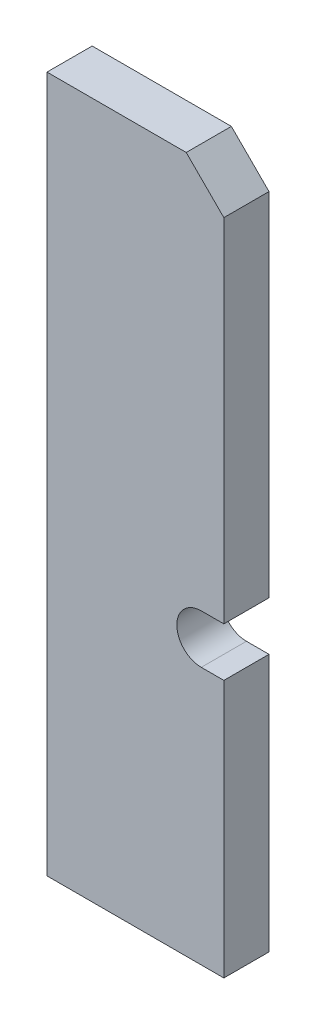
from build123d import *

# Parameters (mm, degrees)
SKETCH_1_W          = 47
SKETCH_1_H          = 185
EXTRUDE_1_DEPTH     = 6
CHAMFER_1_SIZE      = 10
CUT_EXTRUDE_2_REACH = 193.254


with BuildPart() as part:
    # 草图1 → 凸台-拉伸1 (new, symmetric)
    with BuildSketch(Plane.XY):
        with Locations((23.5, 92.5)):
            Rectangle(SKETCH_1_W, SKETCH_1_H)
    extrude(amount=EXTRUDE_1_DEPTH, both=True)

    # 倒角1
    chamfer_1_edges = [part.edges().sort_by_distance(p)[0] for p in [
        (47, 185, 0),
    ]]
    chamfer(chamfer_1_edges, length=CHAMFER_1_SIZE)

    # 草图3 → 切除-拉伸2 (cut, up to next)
    with BuildSketch(Plane(origin=(0, 0, -6), x_dir=(-1, 0, 0), z_dir=(0, 0, -1)), mode=Mode.PRIVATE) as cut_extrude_2_sk1:
        with BuildLine():
            Line((-47, 81.5), (-41, 81.5))
            ThreePointArc((-41, 81.5), (-34.5, 75), (-41, 68.5))
            Line((-41, 68.5), (-47, 68.5))
            Line((-47, 68.5), (-47, 81.5))
        make_face()
    cut_extrude_2_tool1 = extrude(cut_extrude_2_sk1.sketch, amount=-CUT_EXTRUDE_2_REACH, mode=Mode.PRIVATE) & part.part
    add(cut_extrude_2_tool1.solids().sort_by_distance((41.352691, 75, -6))[0], mode=Mode.SUBTRACT)


solid = part.part
